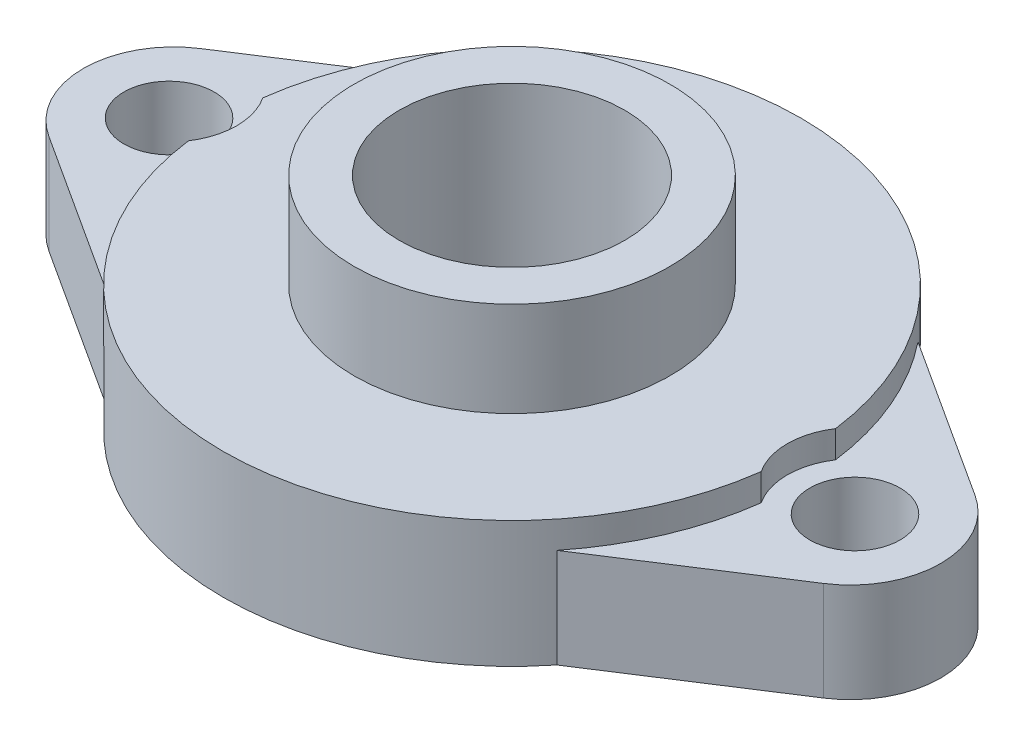
SolidWorks part; units mm, degrees
ref_plane "前视基准面" through (0, 0, 0) normal (0, 0, 1) x (1, 0, 0)
ref_plane "上视基准面" through (0, 0, 0) normal (0, 1, 0) x (1, 0, 0)
ref_plane "右视基准面" through (0, 0, 0) normal (1, 0, 0) x (0, 0, -1)
sketch "草图1" plane through (0, 0, 0) normal (0, 1, 0) x (1, 0, 0)
  circle A0 centre (0, 0) radius 32
  dimension "D1" = 64
extrude "凸台-拉伸1" add sketch "草图1" along normal blind 14
sketch "草图2" plane through (0, 0, 0) normal (0, 1, 0) x (1, 0, 0)
  line L0 (0, 15.8568) -> (0, 0) construction
  line L1 (0, 0) -> (66.8073, 0) construction
  line L2 (42.9285, 8.3983) -> (24.98, 20)
  line L3 (42.9285, -8.3983) -> (24.98, -20)
  arc A0 (42.9285, -8.3983) -> (42.9285, 8.3983) centre (37.5, 0) ccw
  circle A1 centre (0, 0) radius 32 construction
  arc A2 (24.98, -20) -> (24.98, 20) centre (0, 0) ccw
  dimension "D2" = 20
  dimension "D1" = 47.5
  dimension "D3" = 40
extrude "凸台-拉伸2" add sketch "草图2" along normal blind 11
mirror "镜向1" about plane through (0, 0, 0) normal (1, 0, 0) of "凸台-拉伸2"
sketch "草图3" plane through (0, 0, 0) normal (0, 1, 0) x (1, 0, 0)
  line L0 (0, 15.1267) -> (0, 0) construction
  line L1 (0, 0) -> (51.7018, 0) construction
  circle A0 centre (-38, 0) radius 5
  circle A1 centre (38, 0) radius 5
  dimension "D1" = 76
  dimension "D2" = 10
extrude "切除-拉伸1" cut sketch "草图3" along normal through all
sketch "草图4" plane through (0, 14, 0) normal (0, 1, 0) x (1, 0, 0)
  circle A0 centre (-38, 0) radius 7.5
  circle A1 centre (38, 0) radius 7.5
  dimension "D1" = 15
extrude "切除-拉伸2" cut sketch "草图4" against normal up to surface (3 mm away) up to face at (-36.8521, 11, 0)
sketch "草图5" plane through (0, 0, 0) normal (0, 1, 0) x (1, 0, 0)
  circle A0 centre (0, 0) radius 17.5
  dimension "D1" = 35
extrude "凸台-拉伸3" add sketch "草图5" along normal blind 24.5
sketch "草图6" plane through (0, 0, 0) normal (0, -1, 0) x (1, 0, 0)
  circle A0 centre (0, 0) radius 20
  dimension "D1" = 40
extrude "切除-拉伸3" cut sketch "草图6" against normal blind 7
sketch "草图7" plane through (0, 7, 0) normal (0, -1, 0) x (1, 0, 0)
  circle A0 centre (0, 0) radius 17.5
  dimension "D1" = 35
extrude "凸台-拉伸4" add sketch "草图7" along normal blind 3.5
sketch "草图8" plane through (0, 24.5, 0) normal (0, 1, 0) x (1, 0, 0)
  circle A0 centre (0, 0) radius 12.5
  dimension "D1" = 25
extrude "切除-拉伸4" cut sketch "草图8" against normal through all
